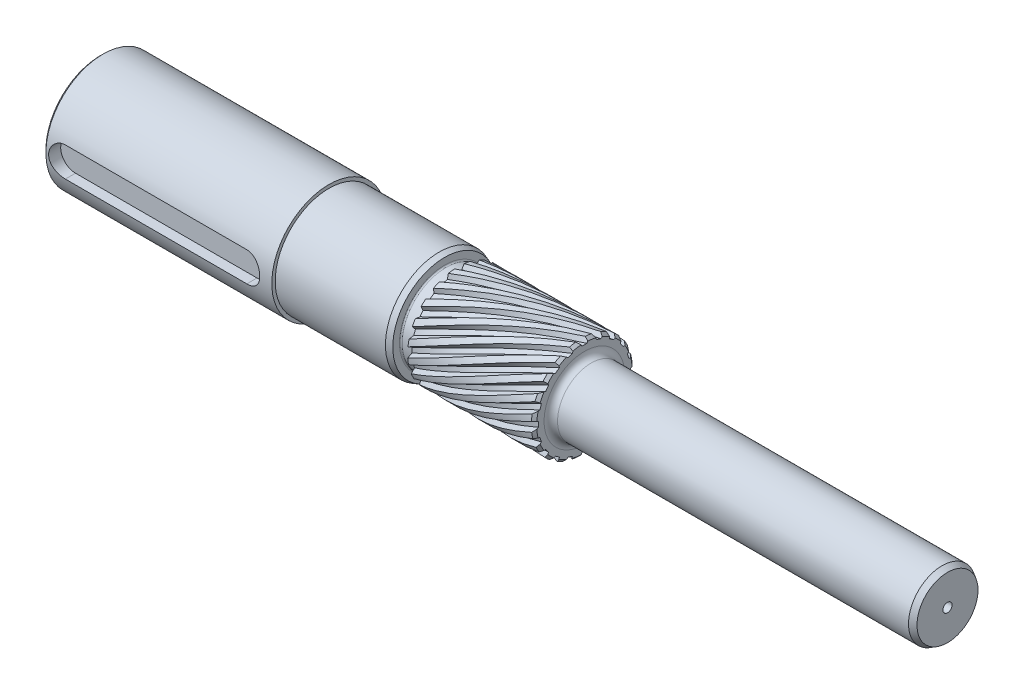
SolidWorks part; units mm, degrees
material "45"
ref_plane "前视基准面" through (0, 0, 0) normal (0, 0, 1) x (1, 0, 0)
ref_plane "上视基准面" through (0, 0, 0) normal (0, 1, 0) x (1, 0, 0)
ref_plane "右视基准面" through (0, 0, 0) normal (1, 0, 0) x (0, 0, -1)
sketch "草图1" plane through (0, 0, 0) normal (1, 0, 0) x (0, 0, -1)
  circle A0 centre (0, 0) radius 42.5
  dimension "D1" = 85
extrude "凸台-拉伸1" add sketch "草图1" along normal blind 360
sketch "草图17" plane through (360, 0, 0) normal (1, 0, 0) x (0, 0, -1)
  circle A0 centre (0, 0) radius 40
  dimension "D1" = 80
extrude "切除-拉伸6" cut sketch "草图17" against normal offset from surface (190 mm away) 170 flip side to cut up to face at (0, 0, -42.5)
sketch "草图3" plane through (360, 0, 0) normal (1, 0, 0) x (0, 0, -1)
  circle A1 centre (0, 0) radius 36
  dimension "D1" = 72
curve "螺旋线/涡状线1" pitch 480 height 94 turns 0.1958
ref_plane "基准面1" through (266, 0, 0) normal (1, 0, 0) x (0, 0, -1)
sketch "草图4" plane through (266, 0, 0) normal (1, 0, 0) x (0, 0, -1)
  circle A0 centre (0, 0) radius 32.5
  dimension "D1" = 65
extrude "切除-拉伸2" cut sketch "草图4" against normal blind 10 flip side to cut
sketch "草图19" plane through (360, 0, 0) normal (1, 0, 0) x (0, 0, -1)
  circle A0 centre (0, 0) radius 37.5
  dimension "D1" = 75
extrude "切除-拉伸7" cut sketch "草图19" against normal up to surface (94 mm away) flip side to cut up to face at (266, 0, -40)
sketch "草图14" plane through (360, 0, 0) normal (1, 0, 0) x (0, 0, -1)
  circle A0 centre (0, 0) radius 42.5
  dimension "D1" = 85
extrude "切除-拉伸4" cut sketch "草图14" against normal up to next (360 mm away) flip side to cut
ref_plane "基准面2" through (0, 0, 42.5) normal (0, 0, 1) x (1, 0, 0)
sketch "草图16" plane through (0, 0, 42.5) normal (0, 0, 1) x (1, 0, 0)
  line L0 (15, 0) -> (150, 0) construction
  line L1 (15, 11) -> (150, 11)
  line L2 (15, -11) -> (150, -11)
  line L3 (0, 42.5) -> (0, -42.5) construction
  arc A0 (15, 11) -> (15, -11) centre (15, 0) ccw
  arc A1 (150, -11) -> (150, 11) centre (150, 0) ccw
  point P3 (82.5, 0)
  dimension "D3" = 15
  dimension "D1" = 22
  dimension "D2" = 135
extrude "切除-拉伸5" cut sketch "草图16" against normal blind 9
chamfer "倒角1" distance 2 angle 45 1 edges at (0, 0, -42.5)
mirror "镜向1" about plane through (0, 0, 0) normal (0, 0, 1) of "切除-拉伸5"
fillet "圆角1" radius 1 2 edges at (266, 0, -32.5) (256, 0, -32.5)
chamfer "倒角2" distance 4 angle 20 1 edges at (256, 0, -40)
sketch "草图20" plane through (0, 0, 0) normal (-1, 0, 0) x (0, 0, 1)
  circle A0 centre (0, 0) radius 25
  dimension "D1" = 50
extrude "凸台-拉伸2" add sketch "草图20" against normal blind 270 from surface at -360 starting at face at (360, 0, -37.5)
chamfer "倒角3" distance 4 angle 30 1 edges at (630, 0, -25)
fillet "圆角2" radius 5 1 edges at (360, 0, -25)
hole_wizard "M8 螺纹孔1" positions "草图24" profile "草图25" tap size "M8" standard "GB"
sketch "草图24" plane through (630, 0, 0) normal (1, 0, 0) x (0, 0, -1)
  point P0 (0, 0)
sketch "草图25" plane through (630, 0, 0) normal (0, 1, 0) x (0, 0, -1)
  line L0 (0, 0) -> (0, 21.7929)
  line L1 (0, 21.7929) -> (3.4, 19.75)
  line L2 (3.4, 19.75) -> (3.4, 0)
  line L5 (3.4, 0) -> (0, 0)
  line L10 (0, 21.7929) -> (-3.4, 19.75) construction
  line L11 (0, -6.35) -> (0, 107.95) construction
  dimension "螺纹孔钻头直径" = 6.8
  dimension "螺纹孔钻头深度" = 19.75
  dimension "导头角度" = 118
cosmetic thread "孔螺蚊线1" parameters "D1"=16, "D2"=8
chamfer "倒角4" distance 2 angle 45 1 edges at (360, 0, -37.5)
sketch "草图26" plane through (360, 0, 0) normal (1, 0, 0) x (0, 0, -1)
  line L0 (0, -1000) -> (0, 49000) construction
  line L1 (-1.7896, 34.25) -> (1.7896, 34.25)
  line L2 (1.7896, 34.25) -> (3.8104, 37.75)
  line L3 (3.8104, 37.75) -> (-3.8104, 37.75)
  line L4 (-3.8104, 37.75) -> (-1.7896, 34.25)
  line L5 (-2.8, 36) -> (2.8, 36) construction
  spline S2 degree 3 poles (0, 36) (-2.1089, 36) (-6.3283, 35.6283) (-12.461, 33.9726) (-18.21, 31.27) (-23.3978, 27.6037) (-27.8645, 23.0865) (-31.4723, 17.8582) (-33.2311, 14.0049) (-33.9351, 12.017) knots 0 0 0 0 0.142857 0.285714 0.428571 0.571429 0.714286 0.857143 1 1 1 1 construction
  point P11 (0, 36)
  dimension "D1" = 5.6
  dimension "D2" = 3.5
  dimension "D3" = 60
sweep "切除-扫描1" cut profiles "草图26" path "螺旋线/涡状线1"
pattern_circular "阵列(圆周)2" count 20 over 360 about axis through (-121.4102, 0, 0) along (1, 0, 0) of "切除-扫描1"
sketch "检测图" plane through (360, 0, 0) normal (1, 0, 0) x (0, 0, -1)
  line L0 (-1.7896, 34.25) -> (-2.462, 35.4145) construction
  line L1 (2.462, 35.4145) -> (1.7896, 34.25) construction
  line L2 (8.8818, 33.1267) -> (8.6022, 34.442) construction
  circle A0 centre (0, 0) radius 36
  point P3 (-2.7397, 35.8956)
  point P7 (2.7397, 35.8956)
  point P8 (8.4867, 34.9854)
  dimension "D1" = 72
equation "\"XMMCDM\"= \"QC名称代码\""
